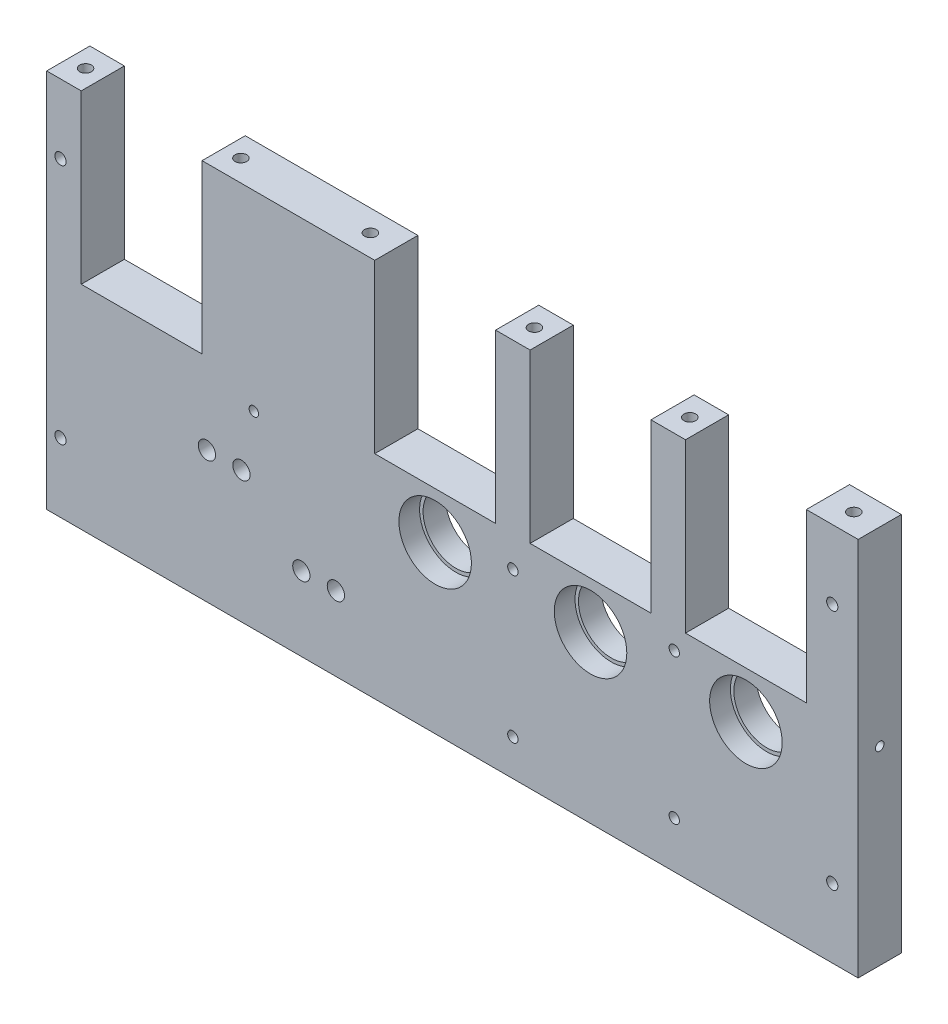
SolidWorks part; units mm, degrees
ref_plane "Front Plane" through (0, 0, 0) normal (0, 0, 1) x (1, 0, 0)
ref_plane "Top Plane" through (0, 0, 0) normal (0, 1, 0) x (1, 0, 0)
ref_plane "Right Plane" through (0, 0, 0) normal (1, 0, 0) x (0, 0, -1)
sketch "Sketch1" plane through (0, 0, 0) normal (0, 0, 1) x (1, 0, 0)
  line L1 (-235, -130) -> (235, -130)
  line L2 (-235, -130) -> (-235, 130)
  line L3 (-235, 130) -> (235, 130)
  line L4 (235, -130) -> (235, 130)
  line L5 (-235, -130) -> (235, 130) construction
  line L6 (-235, 130) -> (235, -130) construction
  point P0 (0, 0)
  dimension "D1" = 470
  dimension "D2" = 260
extrude "Boss-Extrude1" add sketch "Sketch1" along normal mid plane 25
sketch "Sketch4" plane through (0, 0, 12.5) normal (0, 0, 1) x (1, 0, 0)
  line L0 (-215, 130) -> (-215, 33)
  line L1 (235, 130) -> (-235, 130) construction
  line L2 (-215, 33) -> (-145, 33)
  line L3 (-145, 33) -> (-145, 130)
  line L4 (-215, 130) -> (-145, 130)
  line L5 (-45, 130) -> (-45, 33)
  line L6 (-45, 33) -> (25, 33)
  line L7 (25, 33) -> (25, 130)
  line L8 (45, 130) -> (45, 33)
  line L9 (45, 33) -> (115, 33)
  line L10 (115, 33) -> (115, 130)
  line L11 (115, 130) -> (45, 130)
  line L12 (135, 130) -> (135, 33)
  line L13 (135, 33) -> (205, 33)
  line L14 (205, 33) -> (205, 130)
  line L15 (205, 130) -> (135, 130)
  line L17 (235, -130) -> (235, 130) construction
  point P1 (-210, 33.5)
  point P5 (-140, 33.5)
  point P20 (-175, 33.5)
  point P21 (-175, -42.7483)
  point P22 (-195, 33.5)
  point P23 (-195, -42.7483)
  point P24 (-155, 33.5)
  point P25 (-155, -42.7483)
  point P26 (-210, -21.5)
  point P27 (-140, -21.5)
  dimension "D4" = 30
  dimension "D5" = 70
  dimension "D6" = 100
  dimension "D7" = 20
  dimension "D8" = 20
  dimension "D10" = 97
extrude "Cut-Extrude3" cut sketch "Sketch4" against normal blind 97
sketch "Sketch8" plane through (0, 0, 12.5) normal (0, 0, 1) x (1, 0, 0)
  line L0 (-235, -130) -> (235, -130) construction
  line L1 (-318.1638, -90) -> (309.4069, -90)
  line L2 (-318.1638, -90) -> (-318.1638, -194.3749)
  line L3 (-318.1638, -194.3749) -> (309.4069, -194.3749)
  line L4 (309.4069, -90) -> (309.4069, -194.3749)
  dimension "D1" = 40
extrude "Cut-Extrude7" cut sketch "Sketch8" against normal blind 40
hole_wizard "M8 Tapped Hole1" positions "Sketch10" profile "Sketch9" tap size "M8" standard "Gb"
sketch "Sketch10" plane through (0, 130, 0) normal (0, 1, 0) x (1, 0, 0)
  line L0 (-215, 12.5) -> (-235, 12.5) construction
  line L1 (-45, 12.5) -> (-145, 12.5) construction
  line L2 (45, 12.5) -> (25, 12.5) construction
  line L3 (135, 12.5) -> (115, 12.5) construction
  line L4 (235, 12.5) -> (205, 12.5) construction
  line L5 (-235, -12.5) -> (-235, 12.5) construction
  line L6 (-145, 12.5) -> (-145, -12.5) construction
  line L7 (25, 12.5) -> (25, -12.5) construction
  line L8 (115, 12.5) -> (115, -12.5) construction
  line L9 (235, -12.5) -> (235, 12.5) construction
  line L10 (-45, 12.5) -> (-45, -12.5) construction
  point P0 (-225, 0)
  point P2 (-135, 0)
  point P4 (35, 0)
  point P6 (125, 0)
  point P8 (220, 0)
  point P32 (-60, 0)
  dimension "D1" = 12.5
  dimension "D2" = 12.5
  dimension "D3" = 12.5
  dimension "D4" = 12.5
  dimension "D5" = 12.5
  dimension "D6" = 10
  dimension "D7" = 10
  dimension "D8" = 10
  dimension "D9" = 10
  dimension "D10" = 15
  dimension "D11" = 15
  dimension "D12" = 12.5
sketch "Sketch9" plane through (-225, 130, 0) normal (1, 0, 0) x (0, 0, 1)
  line L0 (0, 0) -> (0, 22.0429)
  line L1 (0, 22.0429) -> (3.4, 20)
  line L2 (3.4, 20) -> (3.4, 0)
  line L5 (3.4, 0) -> (0, 0)
  line L10 (0, 22.0429) -> (-3.4, 20) construction
  line L11 (0, -6.35) -> (0, 107.95) construction
  dimension "螺纹孔钻头直径" = 6.8
  dimension "螺纹孔钻头深度" = 20
  dimension "导头角度" = 118
cosmetic thread "Cosmetic Thread1" parameters "D1"=16, "D2"=8
cosmetic thread "Cosmetic Thread2" parameters "D1"=16, "D2"=8
cosmetic thread "Cosmetic Thread3" parameters "D1"=16, "D2"=8
cosmetic thread "Cosmetic Thread4" parameters "D1"=16, "D2"=8
cosmetic thread "Cosmetic Thread5" parameters "D1"=16, "D2"=8
cosmetic thread "Cosmetic Thread11" parameters "D1"=16, "D2"=8
hole_wizard "M10 Tapped Hole1" positions "Sketch16" profile "Sketch15" tap size "M10" standard "Gb"
sketch "Sketch16" plane through (0, -90, 0) normal (0, -1, 0) x (-1, 0, 0)
  line L0 (-235, -12.5) -> (-235, 12.5) construction
  line L1 (235, 12.5) -> (-235, 12.5) construction
  line L2 (235, 12.5) -> (235, -12.5) construction
  point P0 (-155, 0)
  point P2 (155, 0)
  dimension "D1" = 80
  dimension "D2" = 12.5
  dimension "D3" = 80
  dimension "D4" = 12.5
sketch "Sketch15" plane through (155, -90, 0) normal (1, 0, 0) x (0, 0, -1)
  line L0 (0, 0) -> (0, 30.0537)
  line L1 (0, 30.0537) -> (4.25, 27.5)
  line L2 (4.25, 27.5) -> (4.25, 0)
  line L5 (4.25, 0) -> (0, 0)
  line L10 (0, 30.0537) -> (-4.25, 27.5) construction
  line L11 (0, -6.35) -> (0, 107.95) construction
  dimension "螺纹孔钻头直径" = 8.5
  dimension "螺纹孔钻头深度" = 27.5
  dimension "导头角度" = 118
cosmetic thread "Cosmetic Thread9" parameters "D1"=20, "D2"=10
cosmetic thread "Cosmetic Thread10" parameters "D1"=20, "D2"=10
sketch "Sketch17" plane through (0, 0, 12.5) normal (0, 0, 1) x (1, 0, 0)
  line L2 (-45, 33) -> (25, 33) construction
  line L3 (135, 130) -> (135, 33) construction
  line L4 (45, 130) -> (45, 33) construction
  line L5 (-45, 130) -> (-45, 33) construction
  circle A0 centre (170, 6) radius 19
  circle A1 centre (80, 6) radius 19
  circle A2 centre (-10, 6) radius 19
  dimension "D1" = 38
  dimension "D4" = 27
  dimension "D5" = 35
  dimension "D6" = 35
  dimension "D7" = 35
extrude "Cut-Extrude10" cut sketch "Sketch17" against normal through all
sketch "Sketch18" plane through (0, 0, 12.5) normal (0, 0, 1) x (1, 0, 0)
  circle A0 centre (170, 6) radius 21
  circle A1 centre (80, 6) radius 21
  circle A2 centre (-10, 6) radius 21
  dimension "D1" = 42
extrude "Cut-Extrude11" cut sketch "Sketch18" against normal blind 12
sketch "Sketch22" plane through (0, 0, -12.5) normal (0, 0, -1) x (-1, 0, 0)
  line L0 (235, -90) -> (-235, -90) construction
  circle A0 centre (-128.5, 21) radius 3
  circle A1 centre (-128.5, -63) radius 3
  circle A2 centre (-35, 15) radius 3
  circle A3 centre (-35, -69) radius 3
  dimension "D1" = 27
  dimension "D2" = 21
  dimension "D3" = 6
  dimension "D4" = 6
  dimension "D5" = 6
  dimension "D6" = 6
  dimension "D7" = 84
  dimension "D8" = 84
extrude "Cut-Extrude13" cut sketch "Sketch22" against normal through all
sketch "Sketch23" plane through (0, 0, -12.5) normal (0, 0, -1) x (-1, 0, 0)
  line L0 (0, -90) -> (0, 213.9095) construction
  line L1 (235, -90) -> (-235, -90) construction
  line L2 (-235, -90) -> (-235, 130) construction
  line L3 (-235, 130) -> (-205, 130) construction
  circle A0 centre (-220, 90) radius 3.25
  circle A1 centre (-220, -50) radius 3.25
  dimension "D5" = 6.5
  dimension "D1" = 15
  dimension "D2" = 40
  dimension "D3" = 15
  dimension "D4" = 40
extrude "Cut-Extrude14" cut sketch "Sketch23" against normal through all
sketch "Sketch24" plane through (0, 0, -12.5) normal (0, 0, -1) x (-1, 0, 0)
  circle A0 centre (-220, 90) radius 5.5
  circle A1 centre (-220, -50) radius 5.5
  dimension "D1" = 11
extrude "Cut-Extrude15" cut sketch "Sketch24" against normal blind 10
pattern_linear "LPattern1" count 2 spacing 447 along (-1, 0, 0) of "Cut-Extrude14", "Cut-Extrude15"
sketch "Sketch26" plane through (0, 0, -12.5) normal (0, 0, -1) x (-1, 0, 0)
  line L0 (235, -90) -> (-235, -90) construction
  line L1 (235, 130) -> (235, -90) construction
  circle A0 centre (115, 19.25) radius 2.75
  dimension "D1" = 5.5
  dimension "D2" = 109.25
  dimension "D3" = 120
extrude "Cut-Extrude17" cut sketch "Sketch26" against normal through all
sketch "Sketch27" plane through (0, 0, -12.5) normal (0, 0, -1) x (-1, 0, 0)
  circle A0 centre (115, 19.25) radius 5
  dimension "D1" = 10
extrude "Cut-Extrude18" cut sketch "Sketch27" against normal blind 8
sketch "Sketch28" plane through (0, 0, -12.5) normal (0, 0, -1) x (-1, 0, 0)
  circle A0 centre (67.5, -47) radius 5
  circle A1 centre (87.5, -47) radius 5
  circle A2 centre (122.2, -13.8) radius 5
  circle A3 centre (142.2, -13.8) radius 5
  dimension "D1" = 10
extrude "Cut-Extrude19" cut sketch "Sketch28" against normal blind 30
hole_wizard "M6 Tapped Hole1" positions "3DSketch1" profile "Sketch29" tap size "M6" standard "GB"
sketch3d "3DSketch1"
  line L0 (-235, -90, -12.5) -> (-235, -90, 12.5) construction
  line L1 (-235, 130, -12.5) -> (-235, -90, -12.5) construction
  line L2 (235, -90, -12.5) -> (235, 130, -12.5) construction
  line L3 (235, -90, 12.5) -> (235, -90, -12.5) construction
  point P0 (-235, 20, 0)
  point P7 (-235, 20, 0)
  point P9 (235, 20, 0)
  dimension "D1" = 110
  dimension "D2" = 12.5
  dimension "D3" = 12.5
  dimension "D4" = 110
cosmetic thread "Cosmetic Thread12" parameters "D1"=11.5, "D2"=6
sketch "Sketch29" plane through (-235, 20, 0) normal (0, 1, 0) x (0, 0, 1)
  line L0 (0, 0) -> (0, 16.5022)
  line L1 (0, 16.5022) -> (2.5, 15)
  line L2 (2.5, 15) -> (2.5, 0)
  line L5 (2.5, 0) -> (0, 0)
  line L10 (0, 16.5022) -> (-2.5, 15) construction
  line L11 (0, -6.35) -> (0, 107.95) construction
  dimension "螺纹孔钻头直径" = 5
  dimension "螺纹孔钻头深度" = 15
  dimension "导头角度" = 118
cosmetic thread "Cosmetic Thread13" parameters "D1"=11.5, "D2"=6
cosmetic thread "Cosmetic Thread14" parameters "D1"=11.5, "D2"=6
